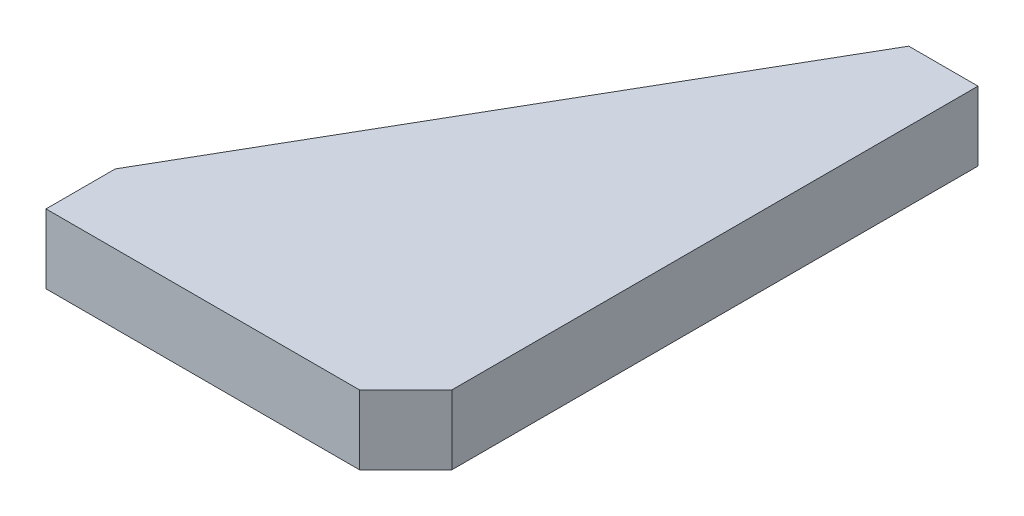
SolidWorks part; units mm, degrees
ref_plane "前视基准面" through (0, 0, 0) normal (0, 0, 1) x (1, 0, 0)
ref_plane "上视基准面" through (0, 0, 0) normal (0, 1, 0) x (1, 0, 0)
ref_plane "右视基准面" through (0, 0, 0) normal (1, 0, 0) x (0, 0, -1)
sketch "草图1" plane through (0, 0, 0) normal (0, 1, 0) x (1, 0, 0)
  line L0 (0, 0) -> (0, -228)
  line L1 (0, -228) -> (-20, -248)
  line L2 (-20, -248) -> (-155.8624, -248)
  line L3 (-155.8624, -248) -> (-155.8624, -218)
  line L4 (-155.8624, -218) -> (-30, 0)
  line L5 (-30, 0) -> (0, 0)
  dimension "D1" = 248
  dimension "D2" = 30
  dimension "D3" = 30
  dimension "D4" = 30
  dimension "D5" = 20
  dimension "D6" = 45
extrude "凸台-拉伸1" add sketch "草图1" along normal blind 30
